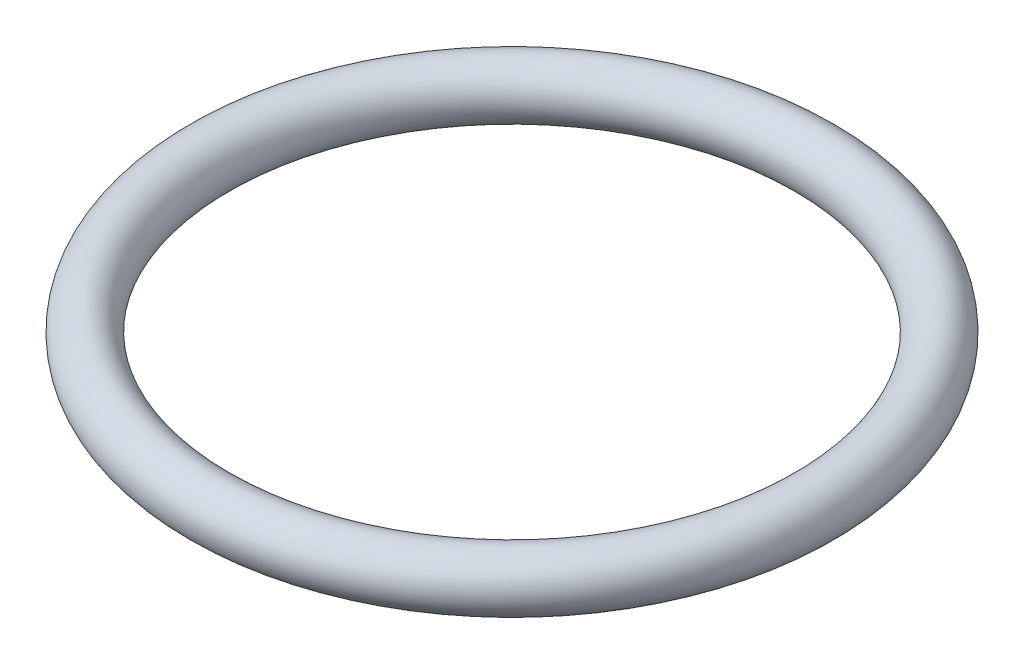
from build123d import *

# Parameters (mm, degrees)
SKETCH1_R = 15


with BuildPart() as part:
    # Sketch1 → Revolve1 (revolve)
    with BuildSketch(Plane.XY, mode=Mode.PRIVATE) as revolve1_sk:
        with Locations((165, 0)):
            Circle(SKETCH1_R)
    revolve(revolve1_sk.sketch.rotate(Axis((0, 0, 0), (0, 1, 0)), 90), axis=Axis((0, 0, 0), (0, 1, 0)))


solid = part.part
